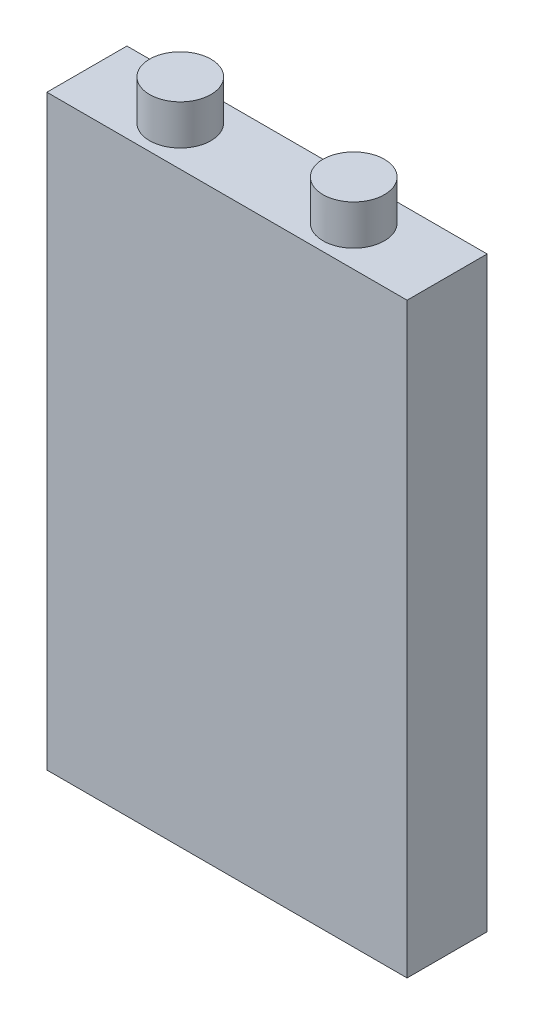
SolidWorks part; units mm, degrees
ref_plane "Front Plane" through (0, 0, 0) normal (0, 0, 1) x (1, 0, 0)
ref_plane "Top Plane" through (0, 0, 0) normal (0, 1, 0) x (1, 0, 0)
ref_plane "Right Plane" through (0, 0, 0) normal (1, 0, 0) x (0, 0, -1)
sketch "Sketch1" plane through (0, 0, 0) normal (0, 0, 1) x (1, 0, 0)
  line L0 (-117.2106, 0) -> (127.4725, 0) construction
  line L1 (0, 96.0453) -> (0, -106.6279) construction
  line L3 (-67.5, 110) -> (67.5, 110)
  line L4 (-67.5, 110) -> (-67.5, -110)
  line L5 (-67.5, -110) -> (67.5, -110)
  line L6 (67.5, 110) -> (67.5, -110)
  dimension "D1" = 135
  dimension "D2" = 220
extrude "Boss-Extrude1" add sketch "Sketch1" along normal mid plane 30
sketch "Sketch2" plane through (0, 110, 0) normal (0, 1, 0) x (1, 0, 0)
  line L0 (-67.5, 0) -> (67.5, 0) construction
  line L1 (-67.5, -15) -> (-67.5, 15) construction
  line L2 (67.5, -15) -> (67.5, 15) construction
  line L3 (0, 15) -> (0, -15) construction
  line L4 (67.5, 15) -> (-67.5, 15) construction
  line L5 (67.5, -15) -> (-67.5, -15) construction
  circle A0 centre (32.5, 0) radius 11.5
  circle A1 centre (-32.5, 0) radius 11.5
  dimension "D1" = 23
  dimension "D2" = 65
extrude "Boss-Extrude2" add sketch "Sketch2" along normal blind 15
